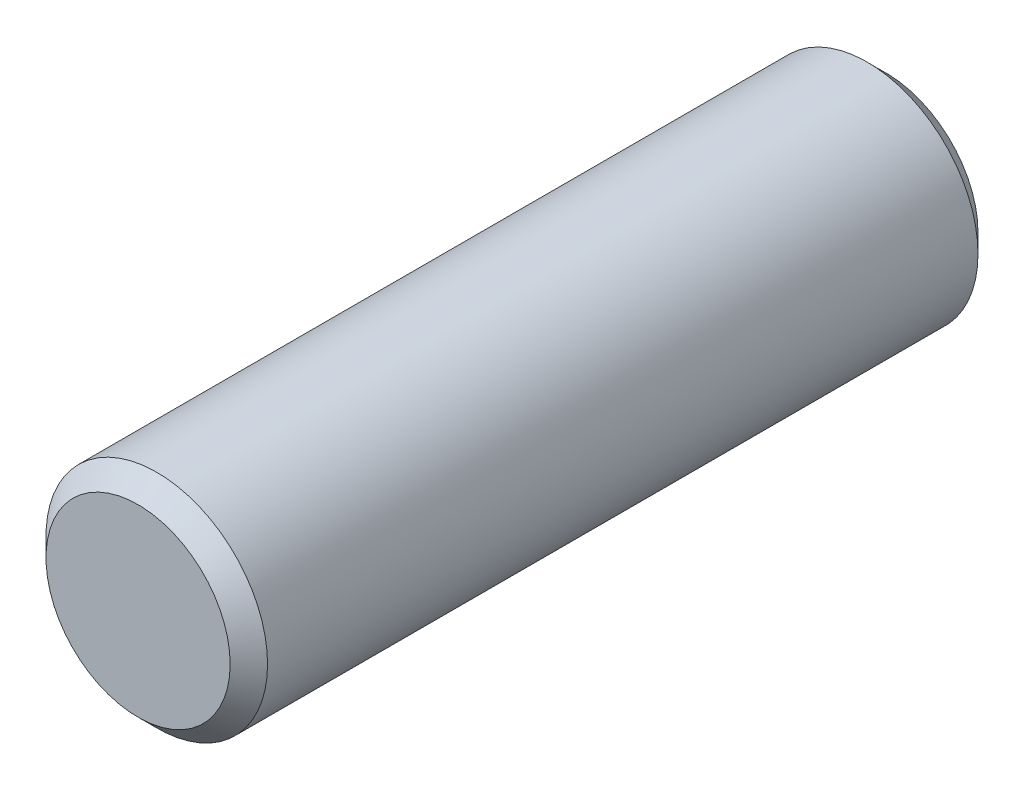
SolidWorks part; units mm, degrees
ref_plane "Front Plane" through (0, 0, 0) normal (0, 0, 1) x (1, 0, 0)
ref_plane "Top Plane" through (0, 0, 0) normal (0, 1, 0) x (1, 0, 0)
ref_plane "Right Plane" through (0, 0, 0) normal (1, 0, 0) x (0, 0, -1)
sketch "Sketch1" plane through (0, 0, 0) normal (0, 0, 1) x (1, 0, 0)
  circle A0 centre (0, 0) radius 5.925
extrude "Boss-Extrude1" add sketch "Sketch1" along normal blind 40
chamfer "Chamfer1" distance 1 distance2 1 2 edges at (5.925, 0, 40) (5.925, 0, 0)
